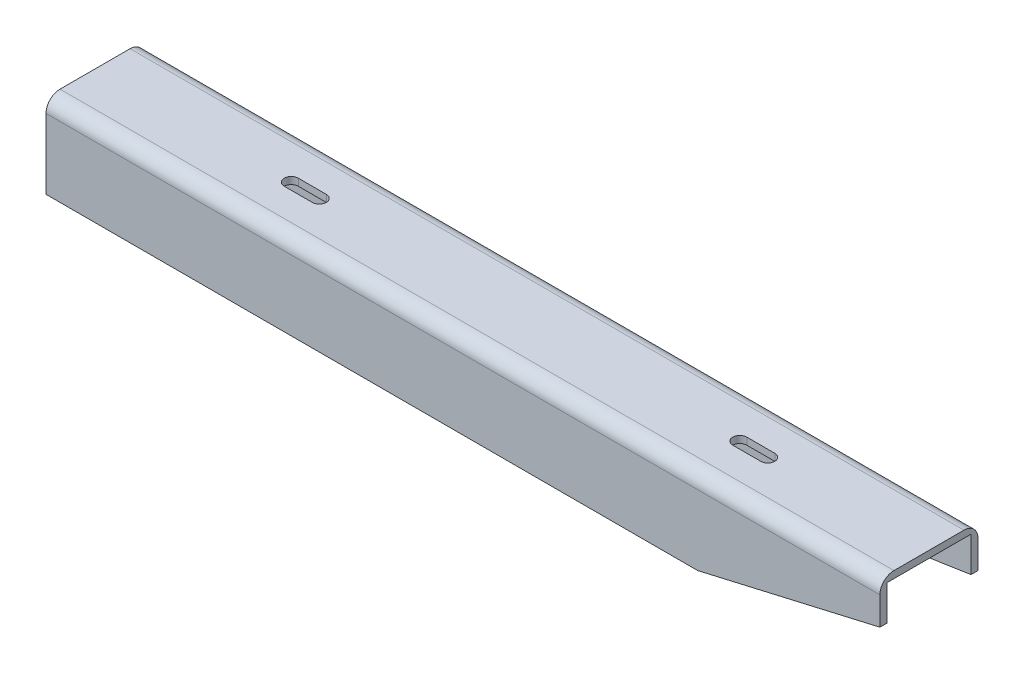
SolidWorks part; units mm, degrees
ref_plane "前视基准面" through (0, 0, 0) normal (0, 0, 1) x (1, 0, 0)
ref_plane "上视基准面" through (0, 0, 0) normal (0, 1, 0) x (1, 0, 0)
ref_plane "右视基准面" through (0, 0, 0) normal (1, 0, 0) x (0, 0, -1)
sketch "草图1" plane through (0, 0, 0) normal (0, 0, 1) x (1, 0, 0)
  line L0 (0, 70) -> (0, -50)
  line L1 (0, 70) -> (570, 70)
  line L2 (570, 70) -> (595, 70)
  line L3 (595, 70) -> (595, 40)
  line L4 (595, 40) -> (0, -50)
extrude "凸台-拉伸1" add sketch "草图1" along normal blind 70
shell "抽壳1" thickness 5
sketch "草图2" plane through (0, 0, 70) normal (0, 0, 1) x (1, 0, 0)
  line L0 (595, 40) -> (0, -50)
  line L1 (0, 70) -> (0, 10)
  line L2 (0, 70) -> (0, -50) construction
  line L3 (0, 10) -> (465, 10)
  line L4 (465, 10) -> (595, 40)
extrude "凸台-拉伸2" add sketch "草图2" against normal blind 5 contours L3 L4 L0
sketch "草图3" plane through (0, 0, 70) normal (0, 0, 1) x (1, 0, 0)
  line L0 (396.6667, 10) -> (-28.7666, 10)
  line L1 (0, -50) -> (0, 10)
  line L2 (0, 70) -> (0, -50) construction
  line L3 (0, -50) -> (396.6667, 10)
  line M2 (0, 70) -> (0, -50)
  line M3 (0, -50) -> (396.6667, 10)
extrude "切除-拉伸1" cut sketch "草图3" against normal blind 5 contours L0 M3 M2
fillet "圆角1" radius 10 1 edges at (297.5, 70, 70)
fillet "圆角2" radius 10 1 edges at (297.5, 70, 0)
sketch "草图4" plane through (0, 70, 0) normal (0, 1, 0) x (1, 0, 0)
  line L0 (140, -30) -> (160, -30)
  line L1 (160, -40) -> (140, -40)
  line L2 (165, -35) -> (455, -35)
  line L3 (485, -35) -> (570, -35)
  line L4 (480, -40) -> (460, -40)
  line L5 (570, -35) -> (595, -35)
  line L6 (460, -30) -> (480, -30)
  arc A0 (140, -30) -> (140, -40) centre (140, -35) ccw
  arc A1 (160, -40) -> (160, -30) centre (160, -35) ccw
  arc A2 (480, -40) -> (480, -30) centre (480, -35) ccw
  arc A3 (460, -30) -> (460, -40) centre (460, -35) ccw
extrude "切除-拉伸2" cut sketch "草图4" against normal blind 5 contours L1 A1 L0 A0 | L6 A3 L4 A2
